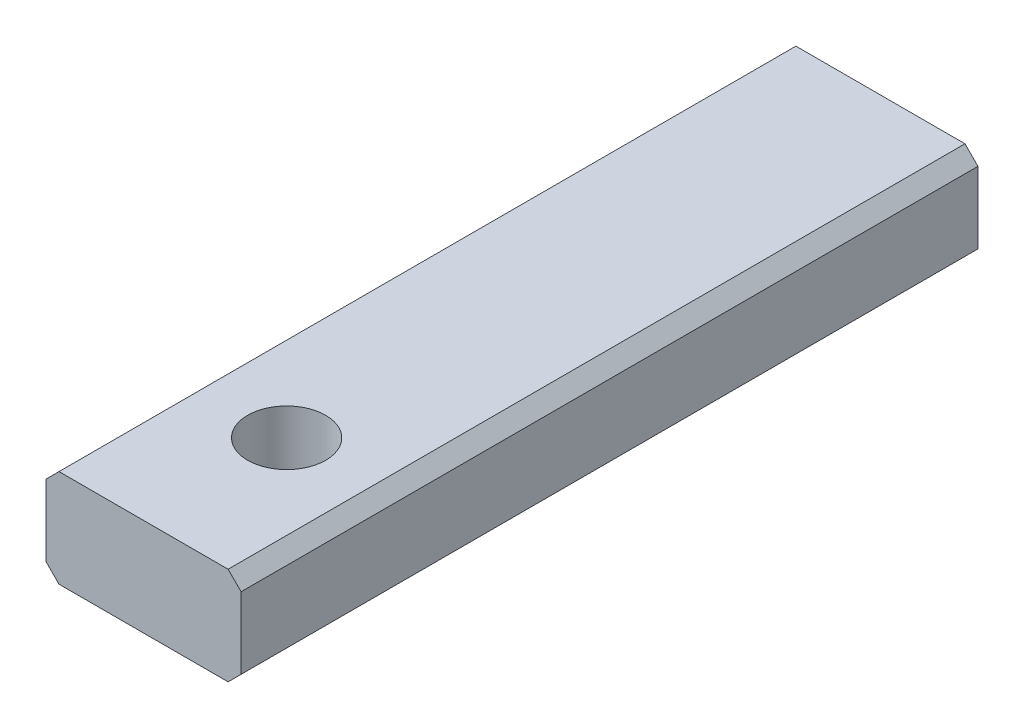
SolidWorks part; units mm, degrees
ref_plane "Front Plane" through (0, 0, 0) normal (0, 0, 1) x (1, 0, 0)
ref_plane "Top Plane" through (0, 0, 0) normal (0, 1, 0) x (1, 0, 0)
ref_plane "Right Plane" through (0, 0, 0) normal (1, 0, 0) x (0, 0, -1)
sketch "Sketch1" plane through (0, 0, 0) normal (0, 0, 1) x (1, 0, 0)
  line L0 (-100, 33.5) -> (-100, 0) construction
  line L1 (-113, 41) -> (-87, 41)
  line L2 (-115, 39) -> (-115, 28)
  line L3 (-113, 26) -> (-87, 26)
  line L4 (-85, 39) -> (-85, 28)
  line L5 (-115, 41) -> (-85, 26) construction
  line L6 (-115, 26) -> (-85, 41) construction
  line L7 (-100, 0) -> (0, 0) construction
  line L8 (-115, 39) -> (-113, 41)
  line L9 (-87, 41) -> (-85, 39)
  line L10 (-85, 28) -> (-87, 26)
  line L11 (-115, 28) -> (-113, 26)
  point P0 (-100, 33.5)
  dimension "D1" = 100
  dimension "D2" = 26
  dimension "D3" = 30
  dimension "D4" = 15
extrude "Boss-Extrude1" add sketch "Sketch1" along normal blind 113.3
sketch "Sketch2" plane through (0, 26, 0) normal (0, -1, 0) x (-1, 0, 0)
  line L0 (100, -113.3) -> (100, -91.3) construction
  line L1 (113, -113.3) -> (87, -113.3) construction
  circle A0 centre (100, -91.3) radius 6
  dimension "D2" = 12
  dimension "D1" = 22
extrude "Cut-Extrude1" cut sketch "Sketch2" against normal blind 110
sketch "Sketch4" plane through (0, 0, 0) normal (0, 0, -1) x (-1, 0, 0)
  line L0 (115, 33.5) -> (100, 33.5) construction
  line L1 (115, 39) -> (115, 28) construction
  line L2 (100, 33.5) -> (100, 41) construction
  line L3 (87, 41) -> (113, 41) construction
  point P1 (100, 33.5)
  point P10 (100, 33.5)
hole_wizard "M8 Tapped Hole 1" positions "Sketch4" profile "Sketch5" tap size "M8" standard "GB"
sketch "Sketch5" plane through (-100, 33.5, 0) normal (1, 0, 0) x (0, 1, 0)
  line L0 (0, 0) -> (0, 19.0429)
  line L1 (0, 19.0429) -> (3.4, 17)
  line L2 (3.4, 17) -> (3.4, 0.625)
  line L3 (3.4, 0.625) -> (4.025, 0)
  line L5 (4.025, 0) -> (0, 0)
  line L6 (-3.4, 0.625) -> (-4.025, 0) construction
  line L10 (0, 19.0429) -> (-3.4, 17) construction
  line L11 (0, -6.35) -> (0, 107.95) construction
  dimension "螺纹孔钻头直径" = 6.8
  dimension "螺纹孔钻头深度" = 17
  dimension "近端锥形沉头孔直径" = 8.05
  dimension "近端锥形沉头孔角度" = 90
  dimension "导头角度" = 118
cosmetic thread "Cosmetic thread 1" parameters "D1"=15, "D2"=8
